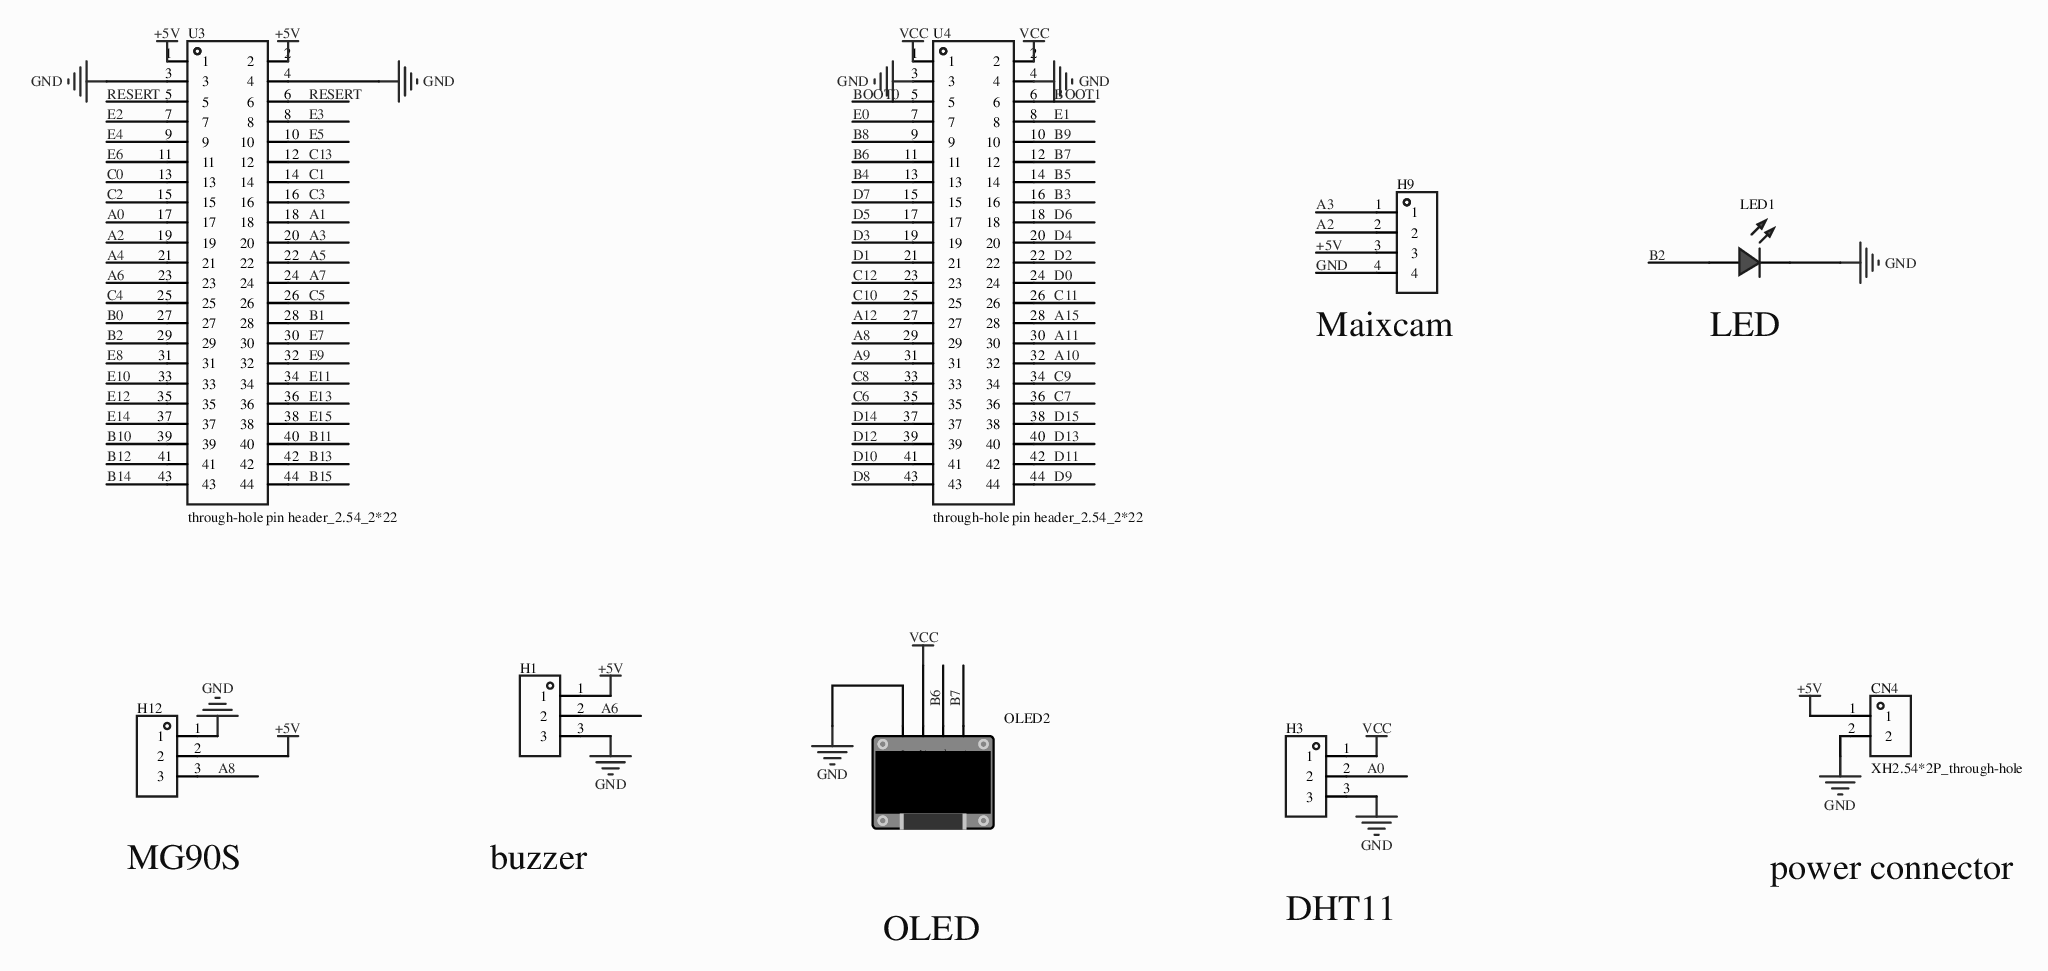
[diagram p0: MISC89054-3.schdoc]
# Altium project MISC89054-2.PrjPcb
1 sheet, 9 parts. Net scope: global (net labels, ports and power ports of the same name join across sheets).
Board file: MISC89054.pcbdoc

## Sheet MISC89054-3.schdoc
size 297 x 209 mm; Version: V1.0; @Project Name: MISC89054; @Page Count: 1; @Update Date: 2026-05-14; @Create Date: 2026-05-14; @Schematic Name: MISC89054; @Page No: 1; @Create Time: 23:22:16; @Update Time: 17:32:40; @Board Name: MISC89054

### Parts
CN4  XH2.54*2P_through-hole  [CONN-TH_2P-P2.50-XH2.54-2P]
H1  (no value)  [HDR-TH_3P-P2.54-V-F]
H3  (no value)  [HDR-TH_3P-P2.54-V-F]
H9  (no value)  [HDR-TH_4P-P2.54-V-F]
H12  (no value)  [HDR-TH_3P-P2.54-V-F]
LED1  (no value)  [LED_TH-3mm]
OLED2  (no value)  [0.96OLED_4P]
U3  through-hole pin header_2.54_2*22  [HDR-TH_44P-P2.54-V-M-R2-C22-S2.54]
U4  through-hole pin header_2.54_2*22  [HDR-TH_44P-P2.54-V-M-R2-C22-S2.54]

### Nets
+5V: CN4.1 H1.1 H9.3 H12.2 U3.1 U3.2
GND: CN4.2 H1.3 H3.3 H9.4 H12.1 LED1.2(A) OLED2.1(GND) U3.3 U3.4 U4.3 U4.4
VCC: H3.1 OLED2.2(VCC) U4.1 U4.2
A0: H3.2 U3.17
A1: U3.18
A2: H9.2 U3.19
A3: H9.1 U3.20
A4: U3.21
A5: U3.22
A6: H1.2 U3.23
A7: U3.24
A8: H12.3 U4.29
A9: U4.31
A10: U4.32
A11: U4.30
A12: U4.27
A15: U4.28
B0: U3.27
B1: U3.28
B2: LED1.1(C) U3.29
B3: U4.16
B4: U4.13
B5: U4.14
B6: OLED2.3(SCL) U4.11
B7: OLED2.4(SDA) U4.12
B8: U4.9
B9: U4.10
B10: U3.39
B11: U3.40
B12: U3.41
B13: U3.42
B14: U3.43
B15: U3.44
BOOT0: U4.5
BOOT1: U4.6
C0: U3.13
C1: U3.14
C2: U3.15
C3: U3.16
C4: U3.25
C5: U3.26
C6: U4.35
C7: U4.36
C8: U4.33
C9: U4.34
C10: U4.25
C11: U4.26
C12: U4.23
C13: U3.12
D0: U4.24
D1: U4.21
D2: U4.22
D3: U4.19
D4: U4.20
D5: U4.17
D6: U4.18
D7: U4.15
D8: U4.43
D9: U4.44
D10: U4.41
D11: U4.42
D12: U4.39
D13: U4.40
D14: U4.37
D15: U4.38
E0: U4.7
E1: U4.8
E2: U3.7
E3: U3.8
E4: U3.9
E5: U3.10
E6: U3.11
E7: U3.30
E8: U3.31
E9: U3.32
E10: U3.33
E11: U3.34
E12: U3.35
E13: U3.36
E14: U3.37
E15: U3.38
RESERT: U3.5 U3.6

### Notes on the sheet
- (near H9) Maixcam
- (near LED1) LED
- (near H12) MG90S
- buzzer
- OLED
- DHT11
- power connector

### Library data of the parts
CN4 = XH2.54*2P_直插: AddInBom: yes; ModelId: 325c595e30db4df8abe76612dd40b0fa0819f05c4eef4c71ace90d822a990e87; ModelTransform: 295.275,228.346,0,180,0,0,-0.002,-20.079,-137.795; Device: XH2.54*2P_through-hole; Symbol: XH2.54*2P_through-hole; FootprintName: CONN-TH_2P-P2.50-XH2.54-2P; LCSC Part Name: XH2.54*2P_直插; SupplierPart: C9900008615; ManufacturerPart: XH2.54*2P_直插; Supplier Footprint: XH2.54_2P; JLCPCB Part Class: Extended Part; Supplier: LCSC; ConvertToPcb: yes; ModelName: CONN-TH_2P-P2.50-XH2.54-2P
H1 H3 H12 = HDR-F_2.54_1x3P: Symbol: PM254V-11-03-H85; ConvertToPcb: yes; ModelId: f3b3cc5aae9641bf9e56fc160cef875b; ModelName: HDR2.54-F-LI-1X3P; ModelTransform: 299.9994,100,0,0,0,0,0,0,-118.11; Device: HDR-F_2.54_1x3P; FootprintName: HDR-TH_3P-P2.54-V-F; AddInBom: yes; SupplierPart: C541850; Supplier Footprint: 插件
H9 = HDR-F_2.54_1x4P: Symbol: 2.54-1*4P female; 3D Model: d187812051054f85879fcaa51a310d8e0819f05c4eef4c71ace90d822a990e87; 3D Model Transform: 419.6842,98.464,0,0,0,0,0,0,-118.11; ConvertToPcb: yes; Device: HDR-F_2.54_1x4P; Supplier Part: C2718488; Supplier Footprint: 插件; FootprintName: HDR-TH_4P-P2.54-V-F; AddInBom: yes; ModelName: HDR-TH_4P-P2.54-V-F
LED1 = LED_TH-R_3mm: ConvertToPcb: yes; ModelId: a497c992633541038a38947cdc58012f0819f05c4eef4c71ace90d822a990e87; ModelName: LED-TH-3mm_R; ModelTransform: 141.274,153.327,0,0,0,0,-5.984,0,-137.795; Symbol: LED_TH-R; Device: LED_TH-R_3mm; AddInBom: yes; FootprintName: LED_TH-3mm; Supplier Footprint: 插件
OLED2 = 0.96OLED模块_4P: Symbol: 0.96OLED module_4P; ConvertToPcb: yes; ModelId: 79c000fdb68d45a296c2e9bedf4f9055; ModelTransform: 1393.69792,1318.895,0,0,0,0,0,-560.079,-137.795; Device: 0.96OLED module_4P; AddInBom: yes; FootprintName: 0.96OLED_4P; Supplier Footprint: 插件; ModelName: 0.96OLED_4P
U3 U4 = 直插排针_2.54_2*22: AddInBom: yes; ModelId: 23a8df7bfd024e7bbe0a3129640493230819f05c4eef4c71ace90d822a990e87; ModelTransform: 2199.99556,196.85,0,0,0,0,0,0,-118.11; Symbol: through-hole pin header_2.54_2*22; Device: through-hole pin header_2.54_2*22; LCSC Part Name: 直插排针_2.54_2*22; SupplierPart: C9900016377; ManufacturerPart: 直插排针_2.54_2*22; Supplier Footprint: P=2.54mm,2*22P，直插; JLCPCB Part Class: Extended Part; Supplier: LCSC; ConvertToPcb: yes; FootprintName: HDR-TH_44P-P2.54-V-M-R2-C22-S2.54; ModelName: HDR-TH_44P-P2.54-V-M-R2-C22-S2.54